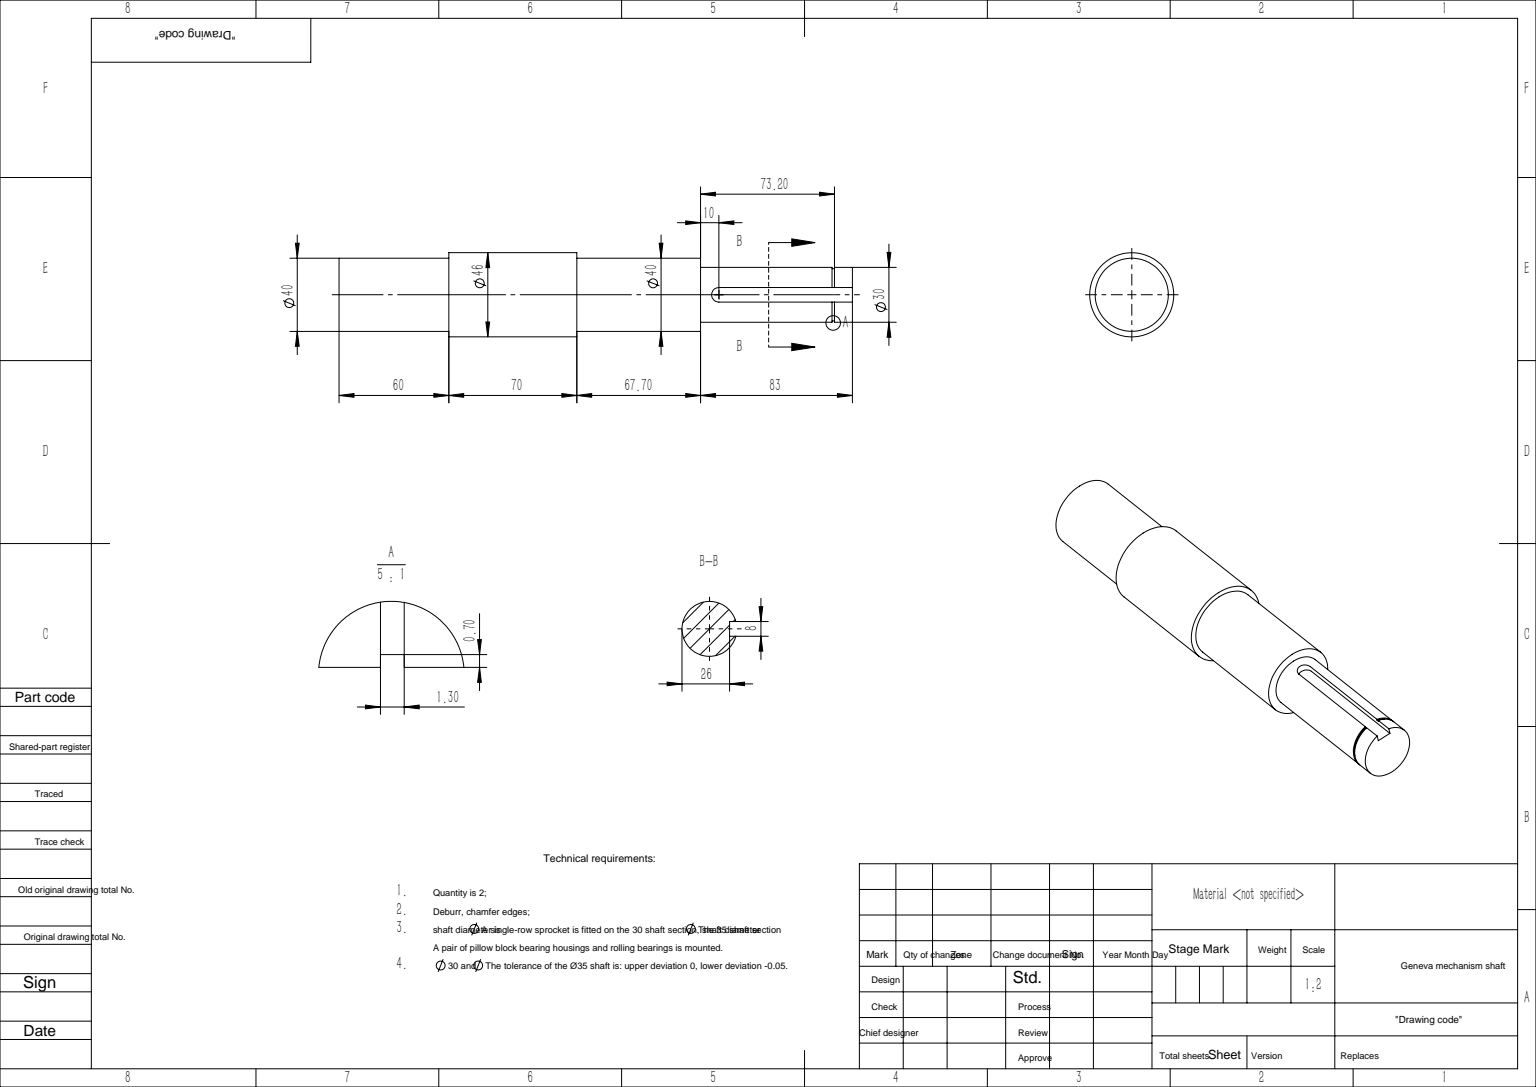
SolidWorks part; units mm, degrees
ref_plane "前视基准面" through (0, 0, 0) normal (0, 0, 1) x (1, 0, 0)
ref_plane "上视基准面" through (0, 0, 0) normal (0, 1, 0) x (1, 0, 0)
ref_plane "右视基准面" through (0, 0, 0) normal (1, 0, 0) x (0, 0, -1)
sketch "草图1" plane through (0, 0, 0) normal (0, 0, 1) x (1, 0, 0)
  line L1 (0, 0) -> (0, 20)
  line L2 (0, 20) -> (60, 20)
  line L3 (60, 20) -> (60, 23)
  line L4 (60, 23) -> (130, 23)
  line L5 (130, 23) -> (130, 20)
  line L6 (130, 20) -> (197.7, 20)
  line L7 (197.7, 20) -> (197.7, 15)
  line L8 (197.7, 15) -> (280.7, 15)
  line L9 (280.7, 15) -> (280.7, 0)
  line L10 (280.7, 0) -> (0, 0)
  dimension "D1" = 20
  dimension "D2" = 60
  dimension "D3" = 23
  dimension "D4" = 70
  dimension "D5" = 20
  dimension "D6" = 67.7
  dimension "D7" = 83
  dimension "D8" = 15
revolve "旋转1" add sketch "草图1" angle 360 about L10
ref_plane "基准面1" through (0, 15, 0) normal (0, 1, 0) x (1, 0, 0)
sketch "草图2" plane through (0, 15, 0) normal (0, 1, 0) x (1, 0, 0)
  line L0 (197.7, 0) -> (280.7, 0) construction
  line L1 (197.7, -20) -> (197.7, 20) construction
  line L2 (280.7, -15) -> (280.7, 15) construction
  line L3 (207.7, 4) -> (290.7, 4)
  line L4 (290.7, 4) -> (290.7, -4)
  line L5 (290.7, -4) -> (207.7, -4)
  arc A0 (207.7, 4) -> (207.7, -4) centre (207.7, 0) ccw
  dimension "D1" = 10
  dimension "D2" = 4
  dimension "D3" = 10
extrude "切除-拉伸1" cut sketch "草图2" against normal blind 4
ref_plane "基准面2" through (270.9, 0, 0) normal (1, 0, 0) x (0, 0, -1)
sketch "草图3" plane through (270.9, 0, 0) normal (1, 0, 0) x (0, 0, -1)
  circle A0 centre (0, 0) radius 14.3
  circle A1 centre (0, 0) radius 15
  circle A2 centre (0, 0) radius 15 construction
  dimension "D1" = 28.6
extrude "切除-拉伸2" cut sketch "草图3" against normal blind 1.3
